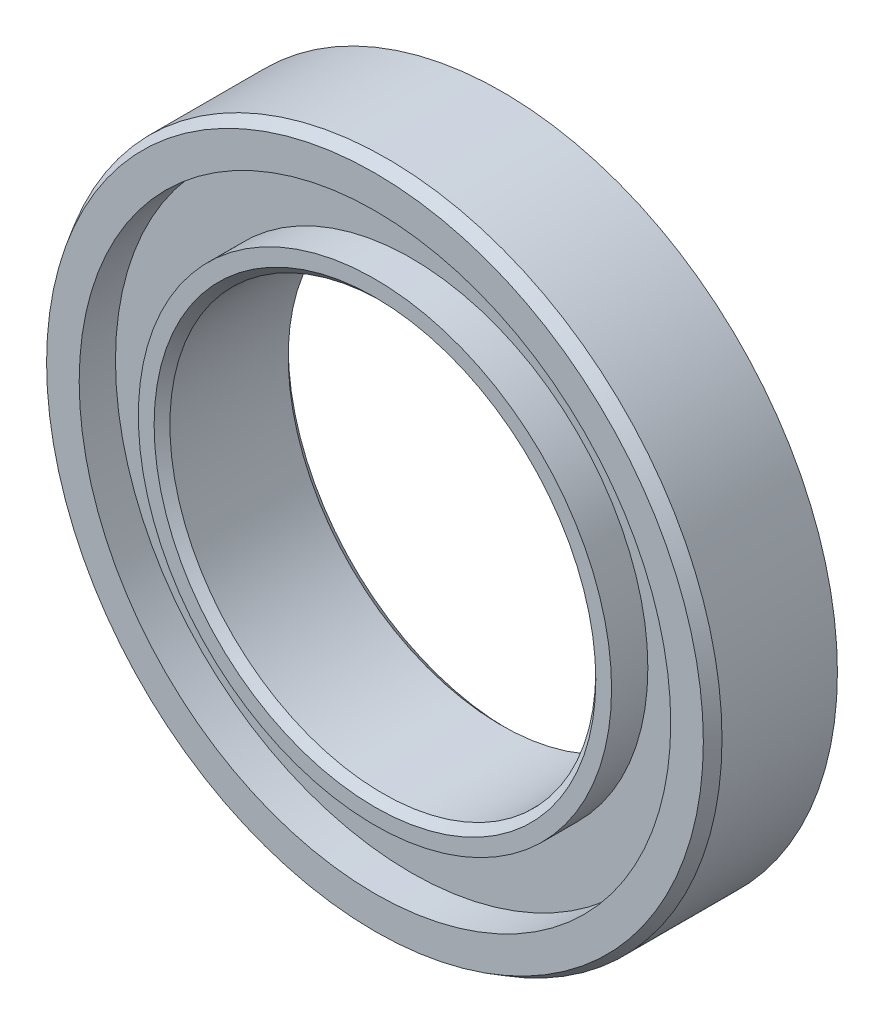
SolidWorks part; units mm, degrees
ref_plane "Front" through (0, 0, 0) normal (0, 0, 1) x (1, 0, 0)
ref_plane "Top" through (0, 0, 0) normal (0, 1, 0) x (1, 0, 0)
ref_plane "Right" through (0, 0, 0) normal (1, 0, 0) x (0, 0, -1)
sketch "Sketch1" plane through (0, 0, 0) normal (0, 0, 1) x (1, 0, 0)
  circle A0 centre (0, 0) radius 42.5
  circle A1 centre (0, 0) radius 27
  dimension "D1" = 85
  dimension "D2" = 54
extrude "Boss-Extrude1" add sketch "Sketch1" along normal blind 17
sketch "Sketch2" plane through (0, 0, 17) normal (0, 0, 1) x (1, 0, 0)
  circle A0 centre (0, 0) radius 37.5
  circle A2 centre (0, 0) radius 30
  dimension "D1" = 75
  dimension "D2" = 7.5
extrude "Cut-Extrude1" cut sketch "Sketch2" against normal blind 4.6
sketch "Sketch3" plane through (0, 0, 0) normal (0, 0, -1) x (-1, 0, 0)
  circle A0 centre (0, 0) radius 37.5
  circle A1 centre (0, 0) radius 30
  dimension "D1" = 75
  dimension "D2" = 7.5
extrude "Cut-Extrude2" cut sketch "Sketch3" against normal blind 4.6
chamfer "Chamfer1" distance 1.5 angle 30 2 edges at (42.5, 0, 17) (42.5, 0, 0)
chamfer "Chamfer2" distance 1 angle 45 2 edges at (27, 0, 0) (27, 0, 17)
equation "\"零件重量\"= IIF ( \"SW-质量\" > 100 , int ( \"SW-质量\" ) , \"SW-质量\" )"
